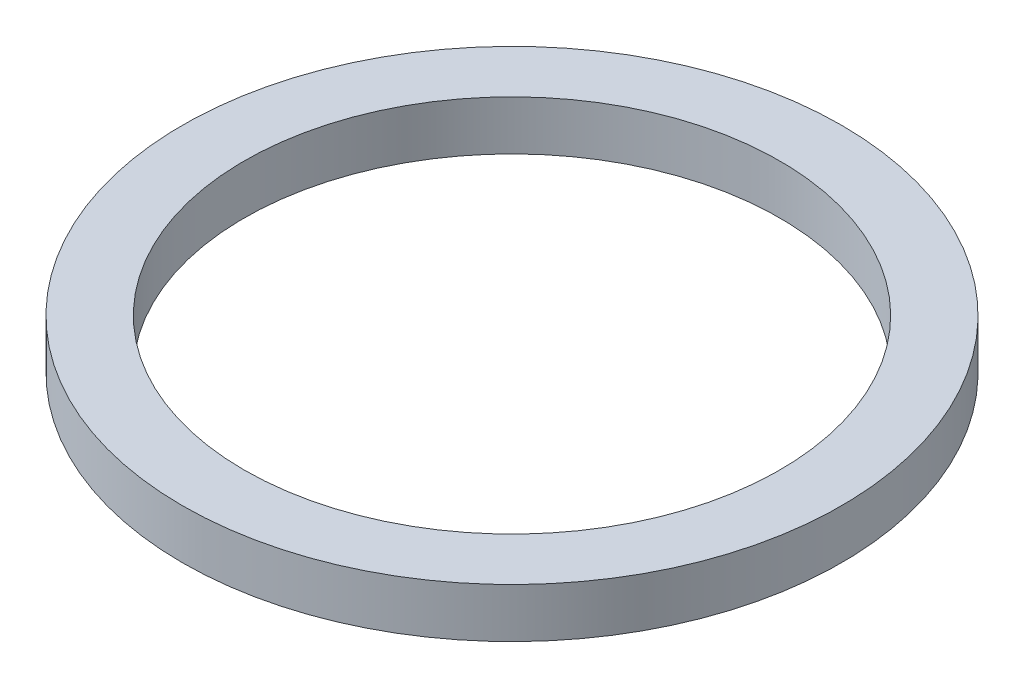
from build123d import *

# Parameters (mm, degrees)
SKETCH1_R           = 40
SKETCH1_R_2         = 32.5
BOSS_EXTRUDE1_DEPTH = 6


with BuildPart() as part:
    # Sketch1 → Boss-Extrude1 (new body)
    with BuildSketch(Plane(origin=(0, 0, 0), x_dir=(1, 0, 0), z_dir=(0, 1, 0))):
        with Locations(Location((0, 0, 0), (0, 0, 270))):
            Circle(SKETCH1_R)
        with Locations(Location((0, 0, 0), (0, 0, 270))):
            Circle(SKETCH1_R_2, mode=Mode.SUBTRACT)
    extrude(amount=BOSS_EXTRUDE1_DEPTH)


solid = part.part
